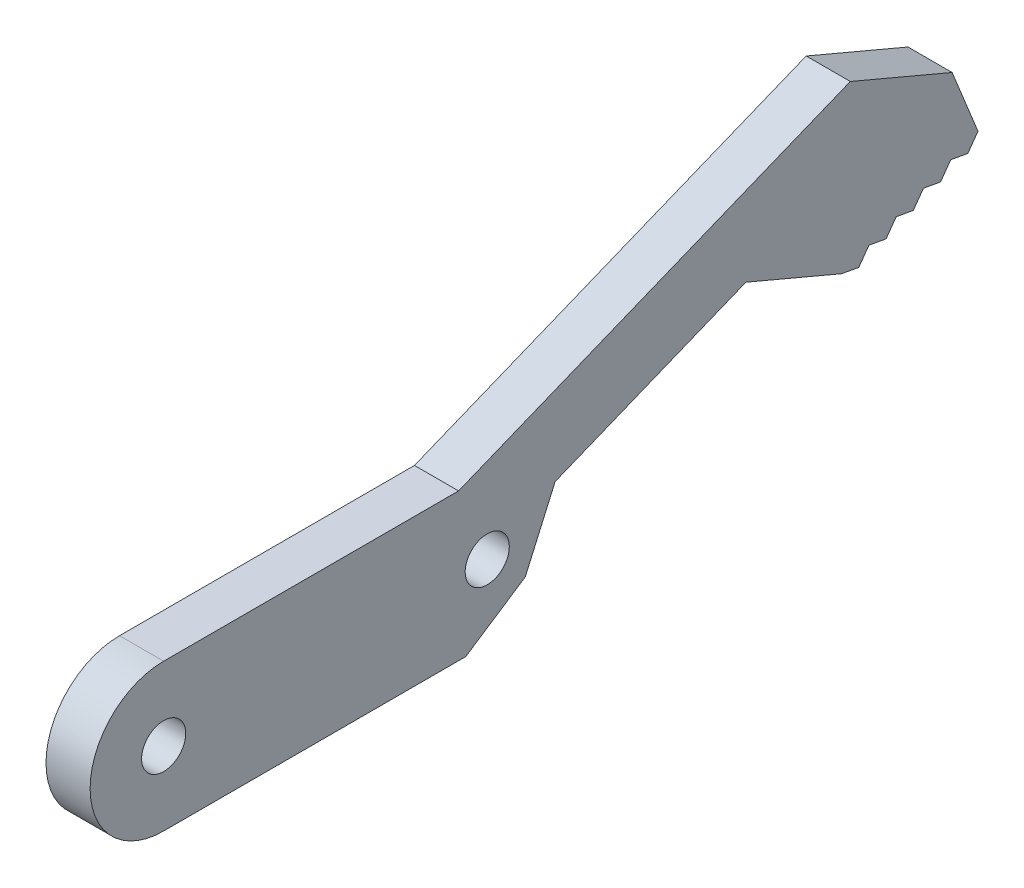
from build123d import *

# Parameters (mm, degrees)
SKETCH1_R           = 5
SKETCH1_R_2         = 1.5
BOSS_EXTRUDE1_DEPTH = 3
BOSS_EXTRUDE2_START = -3
BOSS_EXTRUDE2_DEPTH = 3
CUT_EXTRUDE2_DEPTH  = 65.81382707
CUT_EXTRUDE3_START  = -10
CUT_EXTRUDE3_DEPTH  = 10


with BuildPart() as part:
    # Sketch1 → Boss-Extrude1 (new body)
    # profile 1 of 3: a face of its own
    with BuildSketch(Plane(origin=(0, 0, 0), x_dir=(0, 0, -1), z_dir=(1, 0, 0))):
        with Locations((5, 5)):
            Circle(SKETCH1_R)
        with Locations((5, 5)):
            Circle(SKETCH1_R_2, mode=Mode.SUBTRACT)
    # profile 2 of 3: a face of its own
    with BuildSketch(Plane(origin=(0, 0, 0), x_dir=(0, 0, -1), z_dir=(1, 0, 0))):
        with BuildLine():
            ThreePointArc((10, 5), (8.535533906, 1.464466094), (5, 0))
            Line((5, 0), (27, 0))
            ThreePointArc((27, 0), (22, 5), (27, 10))
            Line((27, 10), (5, 10))
            ThreePointArc((5, 10), (8.535533906, 8.535533906), (10, 5))
        make_face()
    # profile 3 of 3: a face of its own
    with BuildSketch(Plane(origin=(0, 0, 0), x_dir=(0, 0, -1), z_dir=(1, 0, 0))):
        with Locations((27, 5)):
            Circle(SKETCH1_R)
        with Locations((27, 5)):
            Circle(SKETCH1_R_2, mode=Mode.SUBTRACT)
    extrude(amount=BOSS_EXTRUDE1_DEPTH)

    # Sketch2 → Boss-Extrude2 (add)
    with BuildSketch(Plane(origin=(3, 0, 0), x_dir=(0, 0, -1), z_dir=(1, 0, 0)).offset(BOSS_EXTRUDE2_START)):
        with BuildLine():
            ThreePointArc((27, 10), (29.694507461, 9.21184396), (31.53953799, 7.095851816))
            Line((31.53953799, 7.095851816), (31.610157793, 7.262674791))
            Line((31.610157793, 7.262674791), (44.585599673, 12.519851602))
            Line((44.585599673, 12.519851602), (51.097249205, 9.763328363))
            Line((51.097249205, 9.763328363), (60.365421977, 13.518454657))
            Line((60.365421977, 13.518454657), (56.610295683, 22.786627428))
            Line((56.610295683, 22.786627428), (25.051124858, 10))
            Line((25.051124858, 10), (27, 10))
        make_face()
        Polygon((60.365421977, 13.518454657), (51.097249205, 9.763328363), (51.333822162, 9.179433479), (60.601994933, 12.934559772), align=None)
    extrude(amount=BOSS_EXTRUDE2_DEPTH)

    # Sketch4 → Cut-Extrude2 (cut, through all)
    with BuildSketch(Plane(origin=(3, 0, 0), x_dir=(0, 0, -1), z_dir=(1, 0, 0))):
        Polygon((56.610295683, 22.786627428), (51.684261855, 20.790777803), (58.606145308, 17.8605936), align=None)
    extrude(amount=-CUT_EXTRUDE2_DEPTH, mode=Mode.SUBTRACT)

    # Sketch5 → Cut-Extrude3 (cut)
    with BuildSketch(Plane(origin=(3, 0, 0), x_dir=(0, 0, -1), z_dir=(1, 0, 0)).offset(CUT_EXTRUDE3_START)):
        with BuildLine():
            ThreePointArc((27, 0), (31.21184396, 2.305492539), (31.53953799, 7.095851816))
            Line((31.53953799, 7.095851816), (29.583779735, 2.664986829))
            Line((29.583779735, 2.664986829), (25.539598719, 0))
            Line((25.539598719, 0), (27, 0))
        make_face()
        Polygon((52.260639439, 9.554946108), (51.097249205, 9.763328363), (51.333822162, 9.179433479), align=None)
        Polygon((52.95088376, 10.514353622), (52.260639439, 9.554946108), (54.114273993, 10.305971367), align=None)
        Polygon((54.804518314, 11.265378881), (54.114273993, 10.305971367), (55.967908548, 11.056996626), align=None)
        Polygon((56.658152868, 12.01640414), (55.967908548, 11.056996626), (57.821543102, 11.808021884), align=None)
        Polygon((58.511787422, 12.767429398), (57.821543102, 11.808021884), (59.675177656, 12.559047143), align=None)
        Polygon((60.365421977, 13.518454657), (59.675177656, 12.559047143), (60.601994933, 12.934559772), align=None)
    extrude(amount=CUT_EXTRUDE3_DEPTH, mode=Mode.SUBTRACT)


solid = part.part
